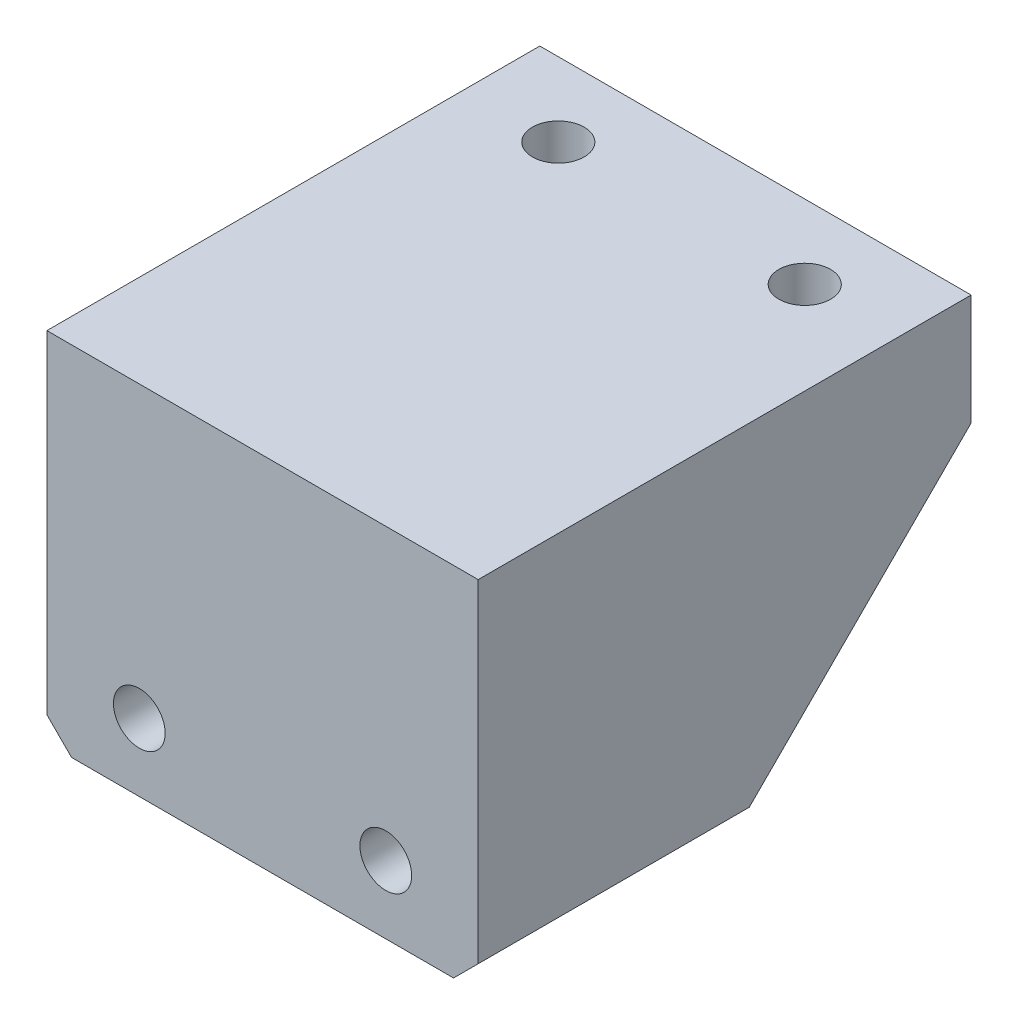
SolidWorks part; units mm, degrees
ref_plane "Front Plane" through (0, 0, 0) normal (0, 0, 1) x (1, 0, 0)
ref_plane "Top Plane" through (0, 0, 0) normal (0, 1, 0) x (1, 0, 0)
ref_plane "Right Plane" through (0, 0, 0) normal (1, 0, 0) x (0, 0, -1)
sketch "Sketch1" plane through (0, 0, 0) normal (0, 1, 0) x (1, 0, 0)
  line L1 (-17.5, 20) -> (17.5, 20)
  line L2 (-17.5, 20) -> (-17.5, -20)
  line L3 (-17.5, -20) -> (17.5, -20)
  line L4 (17.5, 20) -> (17.5, -20)
  line L5 (-17.5, 20) -> (17.5, -20) construction
  line L6 (-17.5, -20) -> (17.5, 20) construction
  point P0 (0, 0)
  dimension "D1" = 35
  dimension "D2" = 40
extrude "Boss-Extrude1" add sketch "Sketch1" along normal blind 29
chamfer "Chamfer1" distance 20 distance2 20 1 edges at (0, 0, -20)
sketch "Sketch2" plane through (0, 0, 20) normal (0, 0, 1) x (1, 0, 0)
  line L0 (0, 0) -> (0, 50000) construction
  line L1 (-17.5, 0) -> (17.5, 0) construction
  point P3 (-10, 5.5)
  point P4 (10, 5.5)
  dimension "D1" = 20
  dimension "D2" = 5.5
hole_wizard "M5 Tapped Hole1" positions "3DSketch1" profile "Sketch3" tap size "M5" standard "Gb"
sketch3d "3DSketch1"
  point P0 (-10, 5.5, 20)
  point P3 (10, 5.5, 20)
sketch "Sketch3" plane through (-10, 5.5, 20) normal (1, 0, 0) x (0, -1, 0)
  line L0 (0, 0) -> (0, 13.6618)
  line L1 (0, 13.6618) -> (2.1, 12.4)
  line L2 (2.1, 12.4) -> (2.1, 0)
  line L5 (2.1, 0) -> (0, 0)
  line L10 (0, 13.6618) -> (-2.1, 12.4) construction
  line L11 (0, -6.35) -> (0, 107.95) construction
  dimension "螺纹孔钻头直径" = 4.2
  dimension "螺纹孔钻头深度" = 12.4
  dimension "导头角度" = 118
cosmetic thread "Cosmetic Thread1"
cosmetic thread "Cosmetic Thread2"
sketch "Sketch4" plane through (0, 29, 0) normal (0, 1, 0) x (1, 0, 0)
  line L0 (0, 0) -> (0, -50000) construction
  line L1 (17.5, 20) -> (-17.5, 20) construction
  point P3 (-10, 14)
  point P4 (10, 14)
  dimension "D1" = 20
  dimension "D2" = 6
hole_wizard "M5 Tapped Hole2" positions "3DSketch2" profile "Sketch6" tap size "M5" standard "Gb" end condition through all
sketch3d "3DSketch2"
  point P0 (-10, 29, -14)
  point P3 (10, 29, -14)
sketch "Sketch6" plane through (-10, 29, -14) normal (1, 0, 0) x (0, 0, 1)
  line L0 (0, 0) -> (0, 29)
  line L1 (0, 29) -> (2.1, 29)
  line L2 (2.1, 29) -> (2.1, 0)
  line L5 (2.1, 0) -> (0, 0)
  line L11 (0, -6.35) -> (0, 107.95) construction
  dimension "通孔螺纹孔钻头直径" = 4.2
  dimension "通孔螺纹孔钻头深度" = 29
cosmetic thread "Cosmetic Thread3"
cosmetic thread "Cosmetic Thread4"
chamfer "Chamfer2" distance 2 angle 45 2 edges at (-17.5, 0, 10) (17.5, 0, 10)
